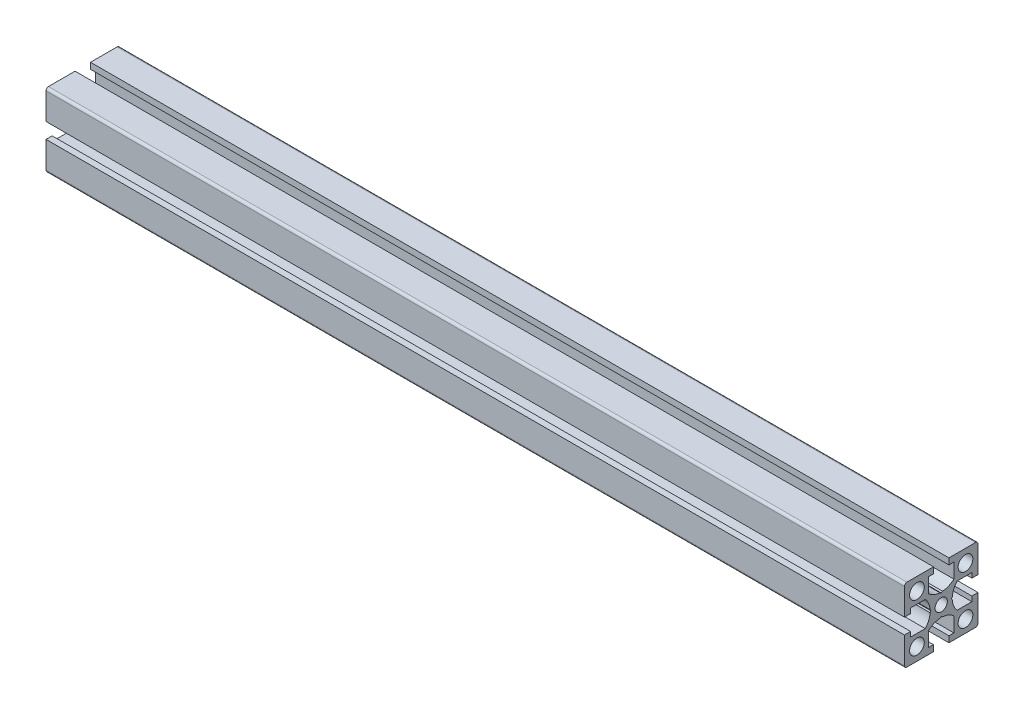
from build123d import *

# Parameters (mm, degrees)
SKETCH_11_R         = 3
SKETCH_11_R_2       = 2.5
F_0_GY_3030_1_DEPTH = 350


with BuildPart() as part:
    # 草图11 → 0国耀铝型材 GY-3030国标铝型材(1) (new body)
    with BuildSketch(Plane.YZ):
        with BuildLine():
            Line((-14, -15), (-3.15, -15))
            Line((-3.15, -15), (-3.15, -12.5))
            Line((-3.15, -12.5), (-5.15, -12.5))
            Line((-5.15, -12.5), (-5.15, -6.5))
            ThreePointArc((-5.15, -6.5), (-3.019390742, -5.122695475), (-0.555, -4.52))
            Line((-0.555, -4.52), (0, -4.2))
            Line((0, -4.2), (0.555, -4.52))
            ThreePointArc((0.555, -4.52), (3.019390742, -5.122695475), (5.15, -6.5))
            Line((5.15, -6.5), (5.15, -12.5))
            Line((5.15, -12.5), (3.15, -12.5))
            Line((3.15, -12.5), (3.15, -15))
            Line((3.15, -15), (14, -15))
            ThreePointArc((14, -15), (14.707106781, -14.707106781), (15, -14))
            Line((15, -14), (15, -3.15))
            Line((15, -3.15), (12.5, -3.15))
            Line((12.5, -3.15), (12.5, -5.15))
            Line((12.5, -5.15), (6.5, -5.15))
            ThreePointArc((6.5, -5.15), (5.12253592, -3.018923167), (4.52, -0.554))
            Line((4.52, -0.554), (4.2, 0))
            Line((4.2, 0), (4.52, 0.555))
            ThreePointArc((4.52, 0.555), (5.122695475, 3.019390742), (6.5, 5.15))
            Line((6.5, 5.15), (12.5, 5.15))
            Line((12.5, 5.15), (12.5, 3.15))
            Line((12.5, 3.15), (15, 3.15))
            Line((15, 3.15), (15, 14))
            ThreePointArc((15, 14), (14.707106781, 14.707106781), (14, 15))
            Line((14, 15), (3.15, 15))
            Line((3.15, 15), (3.15, 12.5))
            Line((3.15, 12.5), (5.15, 12.5))
            Line((5.15, 12.5), (5.15, 6.5))
            ThreePointArc((5.15, 6.5), (3.019292492, 5.123227892), (0.555, 4.521))
            Line((0.555, 4.521), (0, 4.2))
            Line((0, 4.2), (-0.555, 4.521))
            ThreePointArc((-0.555, 4.521), (-3.019292492, 5.123227892), (-5.15, 6.5))
            Line((-5.15, 6.5), (-5.15, 12.5))
            Line((-5.15, 12.5), (-3.15, 12.5))
            Line((-3.15, 12.5), (-3.15, 15))
            Line((-3.15, 15), (-14, 15))
            ThreePointArc((-14, 15), (-14.707106781, 14.707106781), (-15, 14))
            Line((-15, 14), (-15, 3.15))
            Line((-15, 3.15), (-12.5, 3.15))
            Line((-12.5, 3.15), (-12.5, 5.15))
            Line((-12.5, 5.15), (-6.5, 5.15))
            ThreePointArc((-6.5, 5.15), (-5.122695475, 3.019390742), (-4.52, 0.555))
            Line((-4.52, 0.555), (-4.2, 0))
            Line((-4.2, 0), (-4.52, -0.554))
            ThreePointArc((-4.52, -0.554), (-5.12253592, -3.018923167), (-6.5, -5.15))
            Line((-6.5, -5.15), (-12.5, -5.15))
            Line((-12.5, -5.15), (-12.5, -3.15))
            Line((-12.5, -3.15), (-15, -3.15))
            Line((-15, -3.15), (-15, -14))
            ThreePointArc((-15, -14), (-14.707106781, -14.707106781), (-14, -15))
        make_face()
        with Locations((9.8, 9.9)):
            Circle(SKETCH_11_R, mode=Mode.SUBTRACT)
        with Locations((9.8, -9.9)):
            Circle(SKETCH_11_R, mode=Mode.SUBTRACT)
        Circle(SKETCH_11_R_2, mode=Mode.SUBTRACT)
        with Locations((-9.8, 9.9)):
            Circle(SKETCH_11_R, mode=Mode.SUBTRACT)
        with Locations((-10, -9.9)):
            Circle(SKETCH_11_R, mode=Mode.SUBTRACT)
    extrude(amount=F_0_GY_3030_1_DEPTH)


solid = part.part
